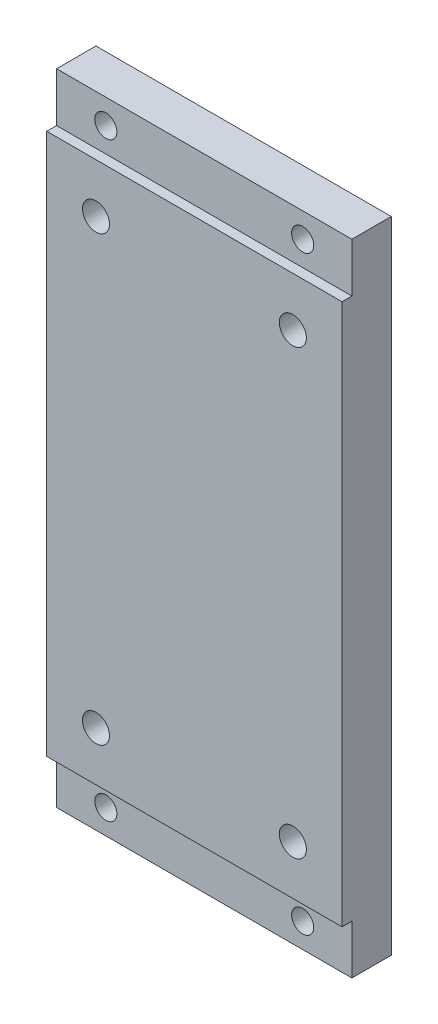
SolidWorks part; units mm, degrees
ref_plane "Front Plane" through (0, 0, 0) normal (0, 0, 1) x (1, 0, 0)
ref_plane "Top Plane" through (0, 0, 0) normal (0, 1, 0) x (1, 0, 0)
ref_plane "Right Plane" through (0, 0, 0) normal (1, 0, 0) x (0, 0, -1)
sketch "Sketch1" plane through (0, 0, 0) normal (0, 0, 1) x (1, 0, 0)
  line L1 (-30, 65) -> (30, 65)
  line L2 (-30, 65) -> (-30, -65)
  line L3 (-30, -65) -> (30, -65)
  line L4 (30, 65) -> (30, -65)
  line L5 (-30, 65) -> (30, -65) construction
  line L6 (-30, -65) -> (30, 65) construction
  point P0 (0, 0)
  dimension "D1" = 60
  dimension "D2" = 130
extrude "Boss-Extrude1" add sketch "Sketch1" along normal blind 10
sketch "Sketch2" plane through (0, 0, 10) normal (0, 0, 1) x (1, 0, 0)
  line L0 (30, -65) -> (30, 65) construction
  line L1 (-30, 65) -> (30, 65)
  line L2 (-30, 65) -> (-30, 55)
  line L3 (-30, 55) -> (30, 55)
  line L4 (30, 65) -> (30, 55)
  line L5 (0, 0) -> (51.627, 0) construction
  line L6 (30, -65) -> (30, -55)
  line L7 (-30, -55) -> (30, -55)
  line L8 (-30, -65) -> (-30, -55)
  line L9 (-30, -65) -> (30, -65)
  dimension "D1" = 10
extrude "Cut-Extrude1" cut sketch "Sketch2" against normal blind 2
hole_wizard "Hole Size by Socket Head Cap Screw Type 1" positions "Sketch4" profile "Sketch3" counterbore size "M4" standard "GB" end condition through all
sketch "Sketch4" plane through (0, 0, 0) normal (0, 0, -1) x (-1, 0, 0)
  point P1 (20, -60)
  point P5 (-20, -60)
  point P9 (20, 60)
  point P13 (-20, 60)
  dimension "D1" = 20
  dimension "D2" = 20
  dimension "D3" = 60
  dimension "D4" = 60
sketch "Sketch3" plane through (-20, -60, 0) normal (1, 0, 0) x (0, 1, 0)
  line L0 (0, 0) -> (0, 10)
  line L1 (0, 10) -> (2.25, 10)
  line L3 (2.25, 10) -> (2.25, 4.6)
  line L4 (2.25, 4.6) -> (4, 4.6)
  line L5 (4, 4.6) -> (4, 0)
  line L7 (4, 0) -> (0, 0)
  line L11 (0, -6.35) -> (0, 107.95) construction
  dimension "通孔孔直径" = 4.5
  dimension "通孔孔深度" = 10
  dimension "柱形沉头孔直径" = 8
  dimension "柱形沉头孔深度" = 4.6
hole_wizard "M5 Clearance Hole1" positions "Sketch6" profile "Sketch5" hole size "M5" standard "GB"
sketch "Sketch6" plane through (0, 0, 10) normal (0, 0, 1) x (1, 0, 0)
  line L1 (0, -45) -> (0, 45) construction
  line L2 (30, -55) -> (30, 55) construction
  line L3 (-30, 55) -> (-30, -55) construction
  line L4 (-30, 55) -> (30, 55) construction
  line L5 (20, -45) -> (20, 45) construction
  line L6 (-20, -45) -> (-20, 45) construction
  line L7 (-30, 0) -> (0, 0) construction
  line L8 (-30, 0) -> (20, 0) construction
  line L9 (-30, 0) -> (-20, 0) construction
  point P13 (20, 45)
  point P14 (20, -45)
  point P15 (-20, 45)
  point P16 (-20, -45)
  dimension "D1" = 10
  dimension "D2" = 10
sketch "Sketch5" plane through (-20, -45, 10) normal (1, 0, 0) x (0, -1, 0)
  line L0 (0, 0) -> (0, 16.6524)
  line L1 (0, 16.6524) -> (2.75, 15)
  line L2 (2.75, 15) -> (2.75, 0)
  line L5 (2.75, 0) -> (0, 0)
  line L10 (0, 16.6524) -> (-2.75, 15) construction
  line L11 (0, -6.35) -> (0, 107.95) construction
  dimension "孔直径" = 5.5
  dimension "孔深度" = 15
  dimension "导头角度" = 118
